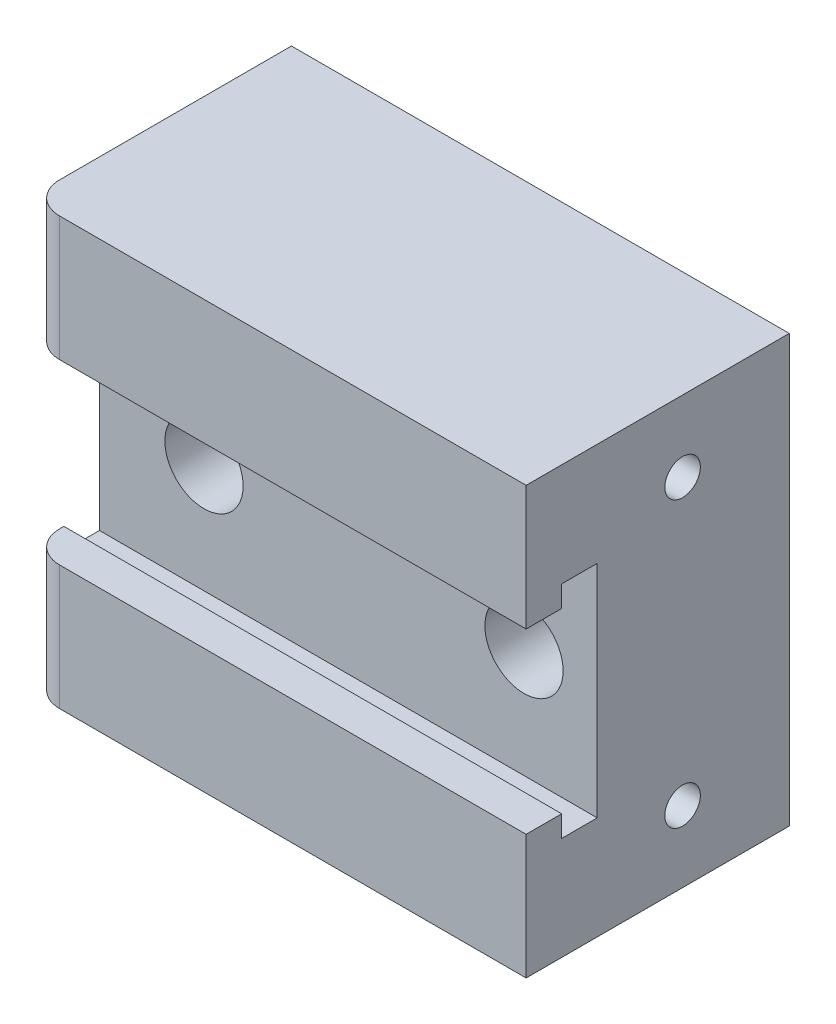
SolidWorks part; units mm, degrees
ref_plane "Front Plane" through (0, 0, 0) normal (0, 0, 1) x (1, 0, 0)
ref_plane "Top Plane" through (0, 0, 0) normal (0, 1, 0) x (1, 0, 0)
ref_plane "Right Plane" through (0, 0, 0) normal (1, 0, 0) x (0, 0, -1)
sketch "Sketch1" plane through (0, 0, 0) normal (0, 0, 1) x (1, 0, 0)
  line L1 (-60.4375, 21.1465) -> (9.5625, 21.1465)
  line L2 (-60.4375, 21.1465) -> (-60.4375, -38.8535)
  line L3 (-60.4375, -38.8535) -> (9.5625, -38.8535)
  line L4 (9.5625, 21.1465) -> (9.5625, -38.8535)
  dimension "D1" = 60
  dimension "D2" = 70
extrude "Boss-Extrude1" add sketch "Sketch1" along normal blind 37
sketch "Sketch3" plane through (9.5625, 0, 0) normal (1, 0, 0) x (0, 0, -1)
  line L1 (-32, -24.3535) -> (-27, -24.3535)
  line L2 (-32, -24.3535) -> (-32, -21.3535)
  line L3 (-32, 6.6465) -> (-27, 6.6465)
  line L4 (-27, -24.3535) -> (-27, 6.6465)
  line L5 (0, -8.8535) -> (-41.4522, -8.8535) construction
  line L6 (0, -38.8535) -> (0, 21.1465) construction
  line L9 (-37, -38.8535) -> (-37, 21.1465) construction
  line L10 (-37, -21.3535) -> (-32, -21.3535)
  line L11 (-37, -21.3535) -> (-37, 3.6465)
  line L12 (-37, 3.6465) -> (-32, 3.6465)
  line L14 (-32, 3.6465) -> (-32, 6.6465)
  dimension "D1" = 31
  dimension "D2" = 5
  dimension "D3" = 27
  dimension "D4" = 25
extrude "Cut-Extrude2" cut sketch "Sketch3" against normal through all
hole_wizard "M6 Tapped Hole1" positions "Sketch6" profile "Sketch5" tap size "M6" standard "ISO"
sketch "Sketch6" plane through (9.5625, 0, 0) normal (1, 0, 0) x (0, 0, -1)
  line L0 (0, -8.8535) -> (-27, -8.8535) construction
  line L1 (0, -38.8535) -> (0, 21.1465) construction
  line L2 (-27, -24.3535) -> (-27, 6.6465) construction
  point P0 (-15, -28.8535)
  point P2 (-15, 11.1465)
  dimension "D1" = 40
  dimension "D2" = 15
sketch "Sketch5" plane through (9.5625, -28.8535, 15) normal (0, 1, 0) x (0, 0, -1)
  line L0 (0, 0) -> (0, 16.5022)
  line L1 (0, 16.5022) -> (2.5, 15)
  line L2 (2.5, 15) -> (2.5, 0)
  line L5 (2.5, 0) -> (0, 0)
  line L10 (0, 16.5022) -> (-2.5, 15) construction
  line L11 (0, -6.35) -> (0, 107.95) construction
  dimension "螺纹孔钻头直径" = 5
  dimension "螺纹孔钻头深度" = 15
  dimension "导头角度" = 118
cosmetic thread "Hole Thread 1" parameters "D1"=12, "D2"=6
cosmetic thread "Hole Thread 2" parameters "D1"=12, "D2"=6
fillet "Fillet1" radius 4.4 2 edges at (-60.4375, 12.3965, 37) (-60.4375, -30.1035, 37)
hole_wizard "CBORE for M6 Hex Socket Head Cap Screw1" positions "Sketch9" profile "Sketch10" counterbore size "M6" standard "ISO" end condition through all
sketch "Sketch9" plane through (0, 0, 37) normal (0, 0, 1) x (1, 0, 0)
  line L0 (9.5625, -8.8535) -> (-60.4375, -8.8535) construction
  line L1 (9.5625, -24.3535) -> (9.5625, 6.6465) construction
  line L2 (-60.4375, -24.3535) -> (-60.4375, 6.6465) construction
  line L3 (-60.4375, -8.8535) -> (-23.2375, 21.1465) construction
  line L4 (9.5625, 21.1465) -> (-56.0375, 21.1465) construction
  line L5 (-23.2375, 21.1465) -> (-23.2375, -38.8535) construction
  line L6 (-56.0375, -38.8535) -> (9.5625, -38.8535) construction
  point P0 (-0.7375, -8.8535)
  point P2 (-45.7375, -8.8535)
  dimension "D1" = 45
sketch "Sketch10" plane through (-0.7375, -8.8535, 37) normal (1, 0, 0) x (0, -1, 0)
  line L0 (0, 0) -> (0, 37)
  line L1 (0, 37) -> (3.3, 37)
  line L3 (3.3, 37) -> (3.3, 25)
  line L4 (3.3, 25) -> (5.5, 25)
  line L5 (5.5, 25) -> (5.5, 0)
  line L7 (5.5, 0) -> (0, 0)
  line L11 (0, -6.35) -> (0, 107.95) construction
  dimension "通孔孔直径" = 6.6
  dimension "通孔孔深度" = 37
  dimension "柱形沉头孔直径" = 11
  dimension "柱形沉头孔深度" = 25
